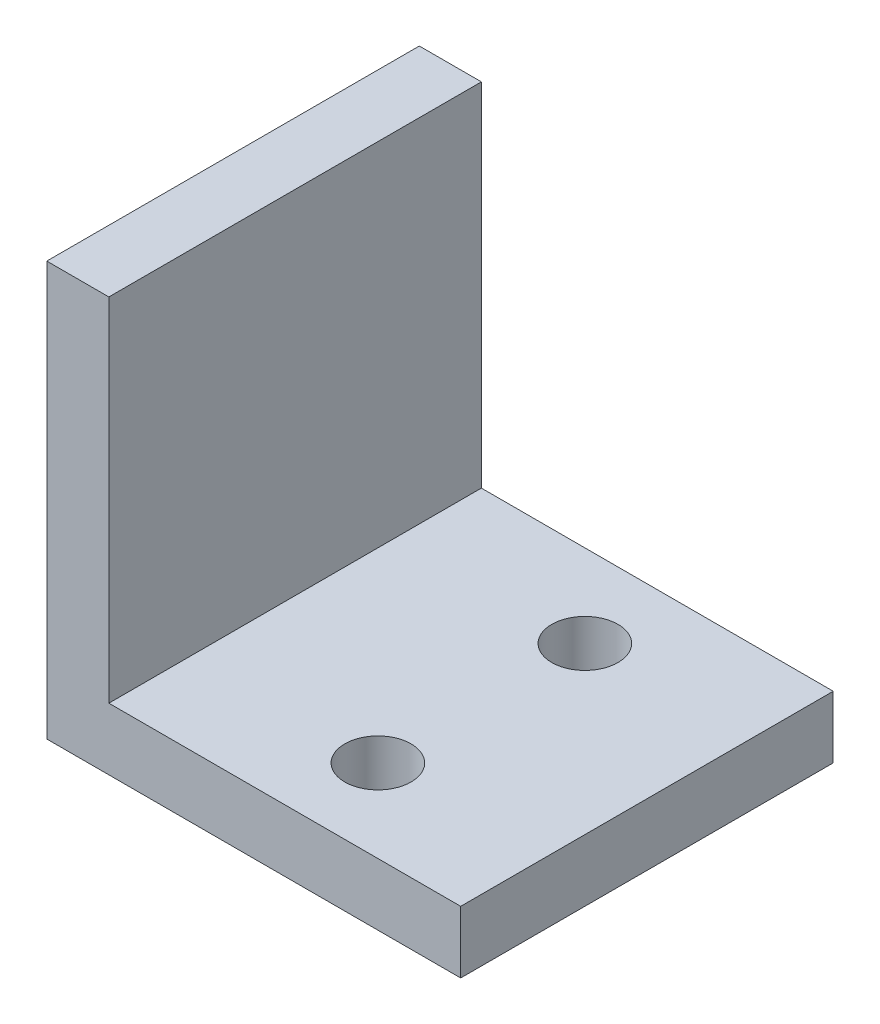
from build123d import *

# Parameters (mm, degrees)
BOSS_EXTRUDE1_DEPTH = 90
SKETCH2_R           = 8
CUT_EXTRUDE1_DEPTH  = 90


with BuildPart() as part:
    # Sketch1 → Boss-Extrude1 (new body)
    with BuildSketch(Plane.XY):
        Polygon((0, 0), (0, 100), (15, 100), (15, 15), (100, 15), (100, 0), align=None)
    extrude(amount=BOSS_EXTRUDE1_DEPTH)

    # Sketch2 → Cut-Extrude1 (cut)
    with BuildSketch(Plane(origin=(0, 15, 0), x_dir=(1, 0, 0), z_dir=(0, 1, 0))):
        with Locations(Location((60, -20, 0), (0, 0, 270))):
            Circle(SKETCH2_R)
        with Locations(Location((60, -70, 0), (0, 0, 270))):
            Circle(SKETCH2_R)
    extrude(amount=-CUT_EXTRUDE1_DEPTH, mode=Mode.SUBTRACT)


solid = part.part
